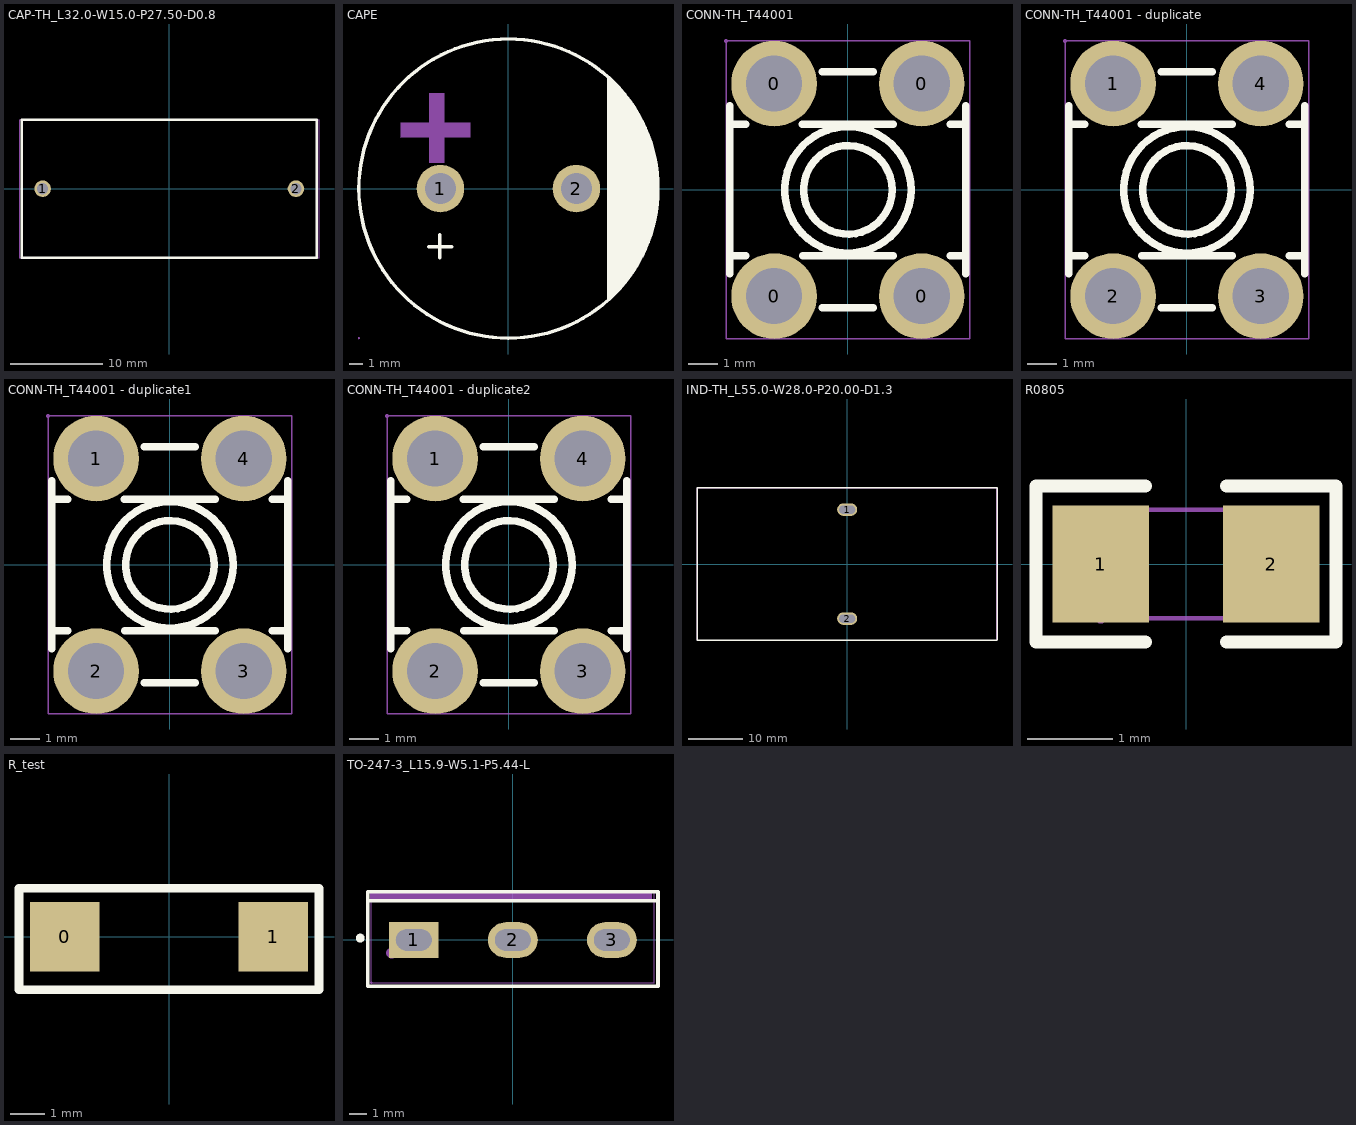
[diagram p0: the footprints below, top view; thin cyan lines are the x and y axes]
# Altium footprint library MISC82254-5.PcbLib: 10 footprints
Each footprint in its own frame and in the unit in brackets; x right, y up, seen from the top. Pads: shape width x height; smd on the part's side, far side on the other; paste and mask are expansions set on the pad; w line width, h text height; cw(c..) or ccw(c..) is an arc to the next point about the centre after c.

## CAP-TH_L32.0-W15.0-P27.50-D0.8 [mm]
pads (2):
  round 1.8 hole 1.2: 1(-13.75,0) 2(13.75,0)
Top Overlay:
  lines w0.254: -16,-7.5 16,-7.5 16,7.5 -16,7.5 -16,-7.5
Mechanical 15:
  region: -16.19,-7.5 -16.19,-7.475 -16.225,-7.44 -16.275,-7.44 -16.31,-7.475 -16.31,-7.5 -16.31,-7.525 -16.275,-7.56 -16.225,-7.56 -16.19,-7.525 -16.19,-7.5
  region: 14.15,0 14.149,0.079 14.087,0.224 13.975,0.335 13.829,0.395 13.671,0.395 13.525,0.335 13.413,0.224 13.351,0.079 13.35,0 13.351,-0.079 13.413,-0.224 13.525,-0.335 13.671,-0.394 13.829,-0.394 13.975,-0.335 14.087,-0.224 14.149,-0.079 14.15,0
  region: -13.35,0 -13.351,0.079 -13.413,0.224 -13.525,0.335 -13.671,0.395 -13.829,0.395 -13.975,0.335 -14.087,0.224 -14.149,0.079 -14.15,0 -14.149,-0.079 -14.087,-0.224 -13.975,-0.335 -13.829,-0.394 -13.671,-0.394 -13.525,-0.335 -13.413,-0.224 -13.351,-0.079 -13.35,0
  lines w0.051: -16.25,-7.5 -16.25,7.5 16.25,7.5 16.25,-7.5 -16.25,-7.5

## CAPE [mm]
pads (2):
  round 3.5 hole 2.3: 1(-5,0) 2(5,0)
Top Overlay:
  circle w0.254: c0,0 r11
  region: 7.28,8.16 7.28,-8.18 7.754,-7.706 8.006,-7.454 8.478,-6.916 8.912,-6.35 9.309,-5.756 9.667,-5.137 9.983,-4.496 10.256,-3.836 10.486,-3.159 10.671,-2.469 10.81,-1.769 10.903,-1.06 10.95,-0.347 10.95,0.01 10.95,0.361 10.904,1.061 10.812,1.757 10.676,2.445 10.494,3.123 10.268,3.788 10,4.436 9.689,5.066 9.338,5.673 8.949,6.257 8.521,6.814 8.059,7.341 7.81,7.59 7.39,8.01
  lines w0.254: -5.842,-4.267 -4.166,-4.267 ; -5.055,-5.105 -5.055,-3.378
Mechanical 6:
  region: -5.808,1.895 -4.758,1.895 -4.733,1.895 -4.727,6.965 -4.733,7.005 -4.738,7.005 -5.797,7.005 -5.833,7.005
  region: -2.82,3.77 -2.82,4.82 -2.82,4.845 -7.89,4.85 -7.93,4.845 -7.93,4.84 -7.93,3.78 -7.93,3.745
Mechanical 15:
  region: -4.1,0 -4.101,0.118 -4.164,0.345 -4.283,0.548 -4.45,0.713 -4.655,0.831 -4.882,0.891 -5.118,0.891 -5.345,0.831 -5.55,0.713 -5.717,0.548 -5.836,0.345 -5.899,0.118 -5.9,0 -5.899,-0.118 -5.836,-0.345 -5.717,-0.548 -5.55,-0.714 -5.345,-0.831 -5.118,-0.891 -4.882,-0.891 -4.655,-0.831 -4.45,-0.714 -4.283,-0.548 -4.164,-0.345 -4.101,-0.118 -4.1,0
  region: 5.9,0 5.899,0.118 5.836,0.345 5.717,0.548 5.55,0.713 5.345,0.831 5.118,0.891 4.882,0.891 4.655,0.831 4.45,0.713 4.283,0.548 4.164,0.345 4.101,0.118 4.1,0 4.101,-0.118 4.164,-0.345 4.283,-0.548 4.45,-0.714 4.655,-0.831 4.882,-0.891 5.118,-0.891 5.345,-0.831 5.55,-0.714 5.717,-0.548 5.836,-0.345 5.899,-0.118 5.9,0
  region: -10.94,-11 -10.94,-10.975 -10.975,-10.94 -11.025,-10.94 -11.06,-10.975 -11.06,-11 -11.06,-11.025 -11.025,-11.06 -10.975,-11.06 -10.94,-11.025 -10.94,-11
  lines w0.051: -11,0 ccw(c0,0) 11,0 ccw(c0,0) -11,0

## CONN-TH_T44001 [mm]
pads (4):
  round 2.9 hole 1.9: 0(-2.5,-3.6) 0(-2.5,3.6) 0(2.5,-3.6) 0(2.5,3.6)
Top Overlay:
  circle w0.254: c0,0 r2.14
  circle w0.254: c0,0 r1.5
  lines w0.254: -4,-2.844 -4,2.844 ; -4,-2.223 -3.463,-2.223 ; -4,2.222 -3.461,2.222 ; -1.539,2.222 1.539,2.222 ; -1.537,-2.223 1.537,-2.223 ; -0.867,-4 0.867,-4 ; -0.867,4 0.867,4 ; 3.461,2.222 4,2.222 ; 3.463,-2.223 4,-2.223 ; 4,-2.844 4,2.844
Mechanical 15:
  region: -4.067,5.05 -4.067,5.075 -4.102,5.11 -4.152,5.11 -4.187,5.075 -4.187,5.05 -4.187,5.025 -4.152,4.99 -4.102,4.99 -4.067,5.025 -4.067,5.05
  region: 3.35,3.6 3.349,3.711 3.29,3.926 3.177,4.118 3.019,4.275 2.826,4.385 2.611,4.443 2.389,4.443 2.174,4.385 1.981,4.275 1.823,4.118 1.71,3.926 1.651,3.711 1.65,3.6 1.651,3.489 1.71,3.274 1.823,3.082 1.981,2.925 2.174,2.815 2.389,2.757 2.611,2.757 2.826,2.815 3.019,2.925 3.177,3.082 3.29,3.274 3.349,3.489 3.35,3.6
  region: 3.35,-3.6 3.349,-3.489 3.29,-3.274 3.177,-3.082 3.019,-2.925 2.826,-2.815 2.611,-2.757 2.389,-2.757 2.174,-2.815 1.981,-2.925 1.823,-3.082 1.71,-3.274 1.651,-3.489 1.65,-3.6 1.651,-3.711 1.71,-3.926 1.823,-4.118 1.981,-4.275 2.174,-4.385 2.389,-4.443 2.611,-4.443 2.826,-4.385 3.019,-4.275 3.177,-4.118 3.29,-3.926 3.349,-3.711 3.35,-3.6
  region: -1.65,-3.6 -1.651,-3.489 -1.71,-3.274 -1.822,-3.082 -1.981,-2.925 -2.174,-2.815 -2.389,-2.757 -2.611,-2.757 -2.826,-2.815 -3.019,-2.925 -3.177,-3.082 -3.29,-3.274 -3.349,-3.489 -3.35,-3.6 -3.349,-3.711 -3.29,-3.926 -3.177,-4.118 -3.019,-4.275 -2.826,-4.385 -2.611,-4.443 -2.389,-4.443 -2.174,-4.385 -1.981,-4.275 -1.823,-4.118 -1.71,-3.926 -1.651,-3.711 -1.65,-3.6
  region: -1.65,3.6 -1.651,3.711 -1.71,3.926 -1.822,4.118 -1.981,4.275 -2.174,4.385 -2.389,4.443 -2.611,4.443 -2.826,4.385 -3.019,4.275 -3.177,4.118 -3.29,3.926 -3.349,3.711 -3.35,3.6 -3.349,3.489 -3.29,3.274 -3.177,3.082 -3.019,2.925 -2.826,2.815 -2.611,2.757 -2.389,2.757 -2.174,2.815 -1.981,2.925 -1.823,3.082 -1.71,3.274 -1.651,3.489 -1.65,3.6
  lines w0.051: -4.127,-5.05 -4.127,5.05 4.127,5.05 4.127,-5.05 -4.127,-5.05

## CONN-TH_T44001 - duplicate [mm]
pads (4):
  round 2.9 hole 1.9: 1(-2.5,3.6) 2(-2.5,-3.6) 3(2.5,-3.6) 4(2.5,3.6)
Top Overlay:
  circle w0.254: c0,0 r1.5
  circle w0.254: c0,0 r2.14
  lines w0.254: -4,-2.844 -4,2.844 ; -4,-2.223 -3.463,-2.223 ; -4,2.222 -3.461,2.222 ; -1.539,2.222 1.539,2.222 ; -1.537,-2.223 1.537,-2.223 ; -0.867,-4 0.867,-4 ; -0.867,4 0.867,4 ; 3.461,2.222 4,2.222 ; 3.463,-2.223 4,-2.223 ; 4,-2.844 4,2.844
Mechanical 15:
  region: -1.65,3.6 -1.651,3.711 -1.71,3.926 -1.822,4.118 -1.981,4.275 -2.174,4.385 -2.389,4.443 -2.611,4.443 -2.826,4.385 -3.019,4.275 -3.177,4.118 -3.29,3.926 -3.349,3.711 -3.35,3.6 -3.349,3.489 -3.29,3.274 -3.177,3.082 -3.019,2.925 -2.826,2.815 -2.611,2.757 -2.389,2.757 -2.174,2.815 -1.981,2.925 -1.823,3.082 -1.71,3.274 -1.651,3.489 -1.65,3.6
  region: -1.65,-3.6 -1.651,-3.489 -1.71,-3.274 -1.822,-3.082 -1.981,-2.925 -2.174,-2.815 -2.389,-2.757 -2.611,-2.757 -2.826,-2.815 -3.019,-2.925 -3.177,-3.082 -3.29,-3.274 -3.349,-3.489 -3.35,-3.6 -3.349,-3.711 -3.29,-3.926 -3.177,-4.118 -3.019,-4.275 -2.826,-4.385 -2.611,-4.443 -2.389,-4.443 -2.174,-4.385 -1.981,-4.275 -1.823,-4.118 -1.71,-3.926 -1.651,-3.711 -1.65,-3.6
  region: 3.35,-3.6 3.349,-3.489 3.29,-3.274 3.177,-3.082 3.019,-2.925 2.826,-2.815 2.611,-2.757 2.389,-2.757 2.174,-2.815 1.981,-2.925 1.823,-3.082 1.71,-3.274 1.651,-3.489 1.65,-3.6 1.651,-3.711 1.71,-3.926 1.823,-4.118 1.981,-4.275 2.174,-4.385 2.389,-4.443 2.611,-4.443 2.826,-4.385 3.019,-4.275 3.177,-4.118 3.29,-3.926 3.349,-3.711 3.35,-3.6
  region: 3.35,3.6 3.349,3.711 3.29,3.926 3.177,4.118 3.019,4.275 2.826,4.385 2.611,4.443 2.389,4.443 2.174,4.385 1.981,4.275 1.823,4.118 1.71,3.926 1.651,3.711 1.65,3.6 1.651,3.489 1.71,3.274 1.823,3.082 1.981,2.925 2.174,2.815 2.389,2.757 2.611,2.757 2.826,2.815 3.019,2.925 3.177,3.082 3.29,3.274 3.349,3.489 3.35,3.6
  region: -4.067,5.05 -4.067,5.075 -4.102,5.11 -4.152,5.11 -4.187,5.075 -4.187,5.05 -4.187,5.025 -4.152,4.99 -4.102,4.99 -4.067,5.025 -4.067,5.05
  lines w0.051: -4.127,-5.05 4.127,-5.05 4.127,5.05 -4.127,5.05 -4.127,-5.05

## CONN-TH_T44001 - duplicate1 [mm]
pads (4):
  round 2.9 hole 1.9: 1(-2.5,3.6) 2(-2.5,-3.6) 3(2.5,-3.6) 4(2.5,3.6)
Top Overlay:
  circle w0.254: c0,0 r2.14
  circle w0.254: c0,0 r1.5
  lines w0.254: -4,-2.844 -4,2.844 ; -4,-2.223 -3.463,-2.223 ; -4,2.222 -3.461,2.222 ; -1.539,2.222 1.539,2.222 ; -1.537,-2.223 1.537,-2.223 ; -0.867,-4 0.867,-4 ; -0.867,4 0.867,4 ; 3.461,2.222 4,2.222 ; 3.463,-2.223 4,-2.223 ; 4,-2.844 4,2.844
Mechanical 15:
  region: -4.067,5.05 -4.067,5.075 -4.102,5.11 -4.152,5.11 -4.187,5.075 -4.187,5.05 -4.187,5.025 -4.152,4.99 -4.102,4.99 -4.067,5.025 -4.067,5.05
  region: 3.35,3.6 3.349,3.711 3.29,3.926 3.177,4.118 3.019,4.275 2.826,4.385 2.611,4.443 2.389,4.443 2.174,4.385 1.981,4.275 1.823,4.118 1.71,3.926 1.651,3.711 1.65,3.6 1.651,3.489 1.71,3.274 1.823,3.082 1.981,2.925 2.174,2.815 2.389,2.757 2.611,2.757 2.826,2.815 3.019,2.925 3.177,3.082 3.29,3.274 3.349,3.489 3.35,3.6
  region: 3.35,-3.6 3.349,-3.489 3.29,-3.274 3.177,-3.082 3.019,-2.925 2.826,-2.815 2.611,-2.757 2.389,-2.757 2.174,-2.815 1.981,-2.925 1.823,-3.082 1.71,-3.274 1.651,-3.489 1.65,-3.6 1.651,-3.711 1.71,-3.926 1.823,-4.118 1.981,-4.275 2.174,-4.385 2.389,-4.443 2.611,-4.443 2.826,-4.385 3.019,-4.275 3.177,-4.118 3.29,-3.926 3.349,-3.711 3.35,-3.6
  region: -1.65,-3.6 -1.651,-3.489 -1.71,-3.274 -1.822,-3.082 -1.981,-2.925 -2.174,-2.815 -2.389,-2.757 -2.611,-2.757 -2.826,-2.815 -3.019,-2.925 -3.177,-3.082 -3.29,-3.274 -3.349,-3.489 -3.35,-3.6 -3.349,-3.711 -3.29,-3.926 -3.177,-4.118 -3.019,-4.275 -2.826,-4.385 -2.611,-4.443 -2.389,-4.443 -2.174,-4.385 -1.981,-4.275 -1.823,-4.118 -1.71,-3.926 -1.651,-3.711 -1.65,-3.6
  region: -1.65,3.6 -1.651,3.711 -1.71,3.926 -1.822,4.118 -1.981,4.275 -2.174,4.385 -2.389,4.443 -2.611,4.443 -2.826,4.385 -3.019,4.275 -3.177,4.118 -3.29,3.926 -3.349,3.711 -3.35,3.6 -3.349,3.489 -3.29,3.274 -3.177,3.082 -3.019,2.925 -2.826,2.815 -2.611,2.757 -2.389,2.757 -2.174,2.815 -1.981,2.925 -1.823,3.082 -1.71,3.274 -1.651,3.489 -1.65,3.6
  lines w0.051: -4.127,-5.05 -4.127,5.05 4.127,5.05 4.127,-5.05 -4.127,-5.05

## CONN-TH_T44001 - duplicate2 [mm]
pads (4):
  round 2.9 hole 1.9: 1(-2.5,3.6) 2(-2.5,-3.6) 3(2.5,-3.6) 4(2.5,3.6)
Top Overlay:
  circle w0.254: c0,0 r2.14
  circle w0.254: c0,0 r1.5
  lines w0.254: -4,-2.844 -4,2.844 ; -4,-2.223 -3.463,-2.223 ; -4,2.222 -3.461,2.222 ; -1.539,2.222 1.539,2.222 ; -1.537,-2.223 1.537,-2.223 ; -0.867,-4 0.867,-4 ; -0.867,4 0.867,4 ; 3.461,2.222 4,2.222 ; 3.463,-2.223 4,-2.223 ; 4,-2.844 4,2.844
Mechanical 15:
  region: -4.067,5.05 -4.067,5.075 -4.102,5.11 -4.152,5.11 -4.187,5.075 -4.187,5.05 -4.187,5.025 -4.152,4.99 -4.102,4.99 -4.067,5.025 -4.067,5.05
  region: 3.35,3.6 3.349,3.711 3.29,3.926 3.177,4.118 3.019,4.275 2.826,4.385 2.611,4.443 2.389,4.443 2.174,4.385 1.981,4.275 1.823,4.118 1.71,3.926 1.651,3.711 1.65,3.6 1.651,3.489 1.71,3.274 1.823,3.082 1.981,2.925 2.174,2.815 2.389,2.757 2.611,2.757 2.826,2.815 3.019,2.925 3.177,3.082 3.29,3.274 3.349,3.489 3.35,3.6
  region: 3.35,-3.6 3.349,-3.489 3.29,-3.274 3.177,-3.082 3.019,-2.925 2.826,-2.815 2.611,-2.757 2.389,-2.757 2.174,-2.815 1.981,-2.925 1.823,-3.082 1.71,-3.274 1.651,-3.489 1.65,-3.6 1.651,-3.711 1.71,-3.926 1.823,-4.118 1.981,-4.275 2.174,-4.385 2.389,-4.443 2.611,-4.443 2.826,-4.385 3.019,-4.275 3.177,-4.118 3.29,-3.926 3.349,-3.711 3.35,-3.6
  region: -1.65,-3.6 -1.651,-3.489 -1.71,-3.274 -1.822,-3.082 -1.981,-2.925 -2.174,-2.815 -2.389,-2.757 -2.611,-2.757 -2.826,-2.815 -3.019,-2.925 -3.177,-3.082 -3.29,-3.274 -3.349,-3.489 -3.35,-3.6 -3.349,-3.711 -3.29,-3.926 -3.177,-4.118 -3.019,-4.275 -2.826,-4.385 -2.611,-4.443 -2.389,-4.443 -2.174,-4.385 -1.981,-4.275 -1.823,-4.118 -1.71,-3.926 -1.651,-3.711 -1.65,-3.6
  region: -1.65,3.6 -1.651,3.711 -1.71,3.926 -1.822,4.118 -1.981,4.275 -2.174,4.385 -2.389,4.443 -2.611,4.443 -2.826,4.385 -3.019,4.275 -3.177,4.118 -3.29,3.926 -3.349,3.711 -3.35,3.6 -3.349,3.489 -3.29,3.274 -3.177,3.082 -3.019,2.925 -2.826,2.815 -2.611,2.757 -2.389,2.757 -2.174,2.815 -1.981,2.925 -1.823,3.082 -1.71,3.274 -1.651,3.489 -1.65,3.6
  lines w0.051: -4.127,-5.05 -4.127,5.05 4.127,5.05 4.127,-5.05 -4.127,-5.05

## IND-TH_L55.0-W28.0-P20.00-D1.3 [mm]
pads (2):
  oval 3.7x2.3 hole 1.5 slot 2.9 at 0 deg paste+0 mask+0.05: 1(0,10) 2(0,-10)
Top Overlay:
  lines w0.254: -27.5,-14 -27.5,14 27.5,14 27.5,-14 -27.5,-14
Mechanical 15:
  region: -1,10.5 1,10.5 1,9.5 -1,9.5
  region: -1,-9.5 1,-9.5 1,-10.5 -1,-10.5
  region: -27.44,14 -27.44,14.025 -27.475,14.06 -27.525,14.06 -27.56,14.025 -27.56,14 -27.56,13.975 -27.525,13.94 -27.475,13.94 -27.44,13.975 -27.44,14
  lines w0.051: -27.5,-14 27.5,-14 27.5,14 -27.5,14 -27.5,-14

## R0805 [mm]
pads (2):
  rect 1.133x1.377 smd paste-100 mask+0.051: 1(-1,0) 2(1,0)
Top Overlay:
  lines w0.152: -0.476,-0.917 -1.761,-0.917 -1.761,0.917 -0.476,0.917 ; 0.476,-0.917 1.761,-0.917 1.761,0.917 0.476,0.917
Top Paste:
  region: 0.45,-0.64 0.45,-0.22 0.895,-0.22 0.895,0.23 0.455,0.23 0.45,0.64 0.5,0.69 1.65,0.69 1.7,0.64 1.7,-0.64 1.65,-0.69 0.5,-0.69
  region: -1.7,-0.64 -1.7,0.64 -1.65,0.69 -0.5,0.69 -0.45,0.64 -0.445,0.23 -0.895,0.23 -0.895,-0.22 -0.455,-0.22 -0.45,-0.64 -0.5,-0.69 -1.65,-0.69
Mechanical 15:
  region: -0.94,-0.638 -0.941,-0.614 -0.976,-0.58 -1.024,-0.58 -1.059,-0.613 -1.06,-0.637 -1.059,-0.661 -1.024,-0.695 -0.976,-0.695 -0.941,-0.662 -0.94,-0.638
  region: 1,-0.637 1,0.637 0.6,0.637 0.6,-0.637
  region: -1,-0.637 -1,0.637 -0.6,0.637 -0.6,-0.637
  lines w0.051: -1,-0.637 1,-0.637 1,0.637 -1,0.637 -1,-0.637

## R_test [mm]
pads (2):
  rect 2x2 smd: 0(-3,0) 1(3,0)
Top Overlay:
  lines w0.254: -4.318,-1.524 -4.318,1.397 4.318,1.397 4.318,-1.524 -4.318,-1.524

## TO-247-3_L15.9-W5.1-P5.44-L [mm]
pads (3):
  rect 2.8x2 hole 1.2 slot 2 at 0 deg: 1(-5.56,0)
  oval 2.8x2 hole 1.2 slot 2 at 0 deg: 2(0,0) 3(5.56,0)
Top Overlay:
  lines w0.201: -8.151,2.2 8.151,2.2 ; -8.151,-2.601 8.151,-2.601 8.151,2.7 -8.151,2.7 -8.151,-2.601
  lines w0.249: -8.57,0.23 ccw(c-8.569,0.106) -8.567,0.23
Mechanical 6:
  circle w0.3: c-6.81,-0.73 r0.15
  region: -8.005,2.24 -8.005,2.71 7.805,2.71 7.805,2.24
Mechanical 15:
  region: -7.89,-2.39 -7.891,-2.366 -7.926,-2.332 -7.974,-2.332 -8.009,-2.366 -8.01,-2.39 -8.009,-2.414 -7.974,-2.448 -7.926,-2.448 -7.891,-2.414 -7.89,-2.39
  region: 6.16,0.3 6.16,-0.3 4.96,-0.3 4.96,0.3
  region: 0.6,0.3 0.6,-0.3 -0.6,-0.3 -0.6,0.3
  region: -4.96,0.3 -4.96,-0.3 -6.16,-0.3 -6.16,0.3
  lines w0.051: -7.95,-2.39 7.95,-2.39 7.95,2.71 -7.95,2.71 -7.95,-2.39